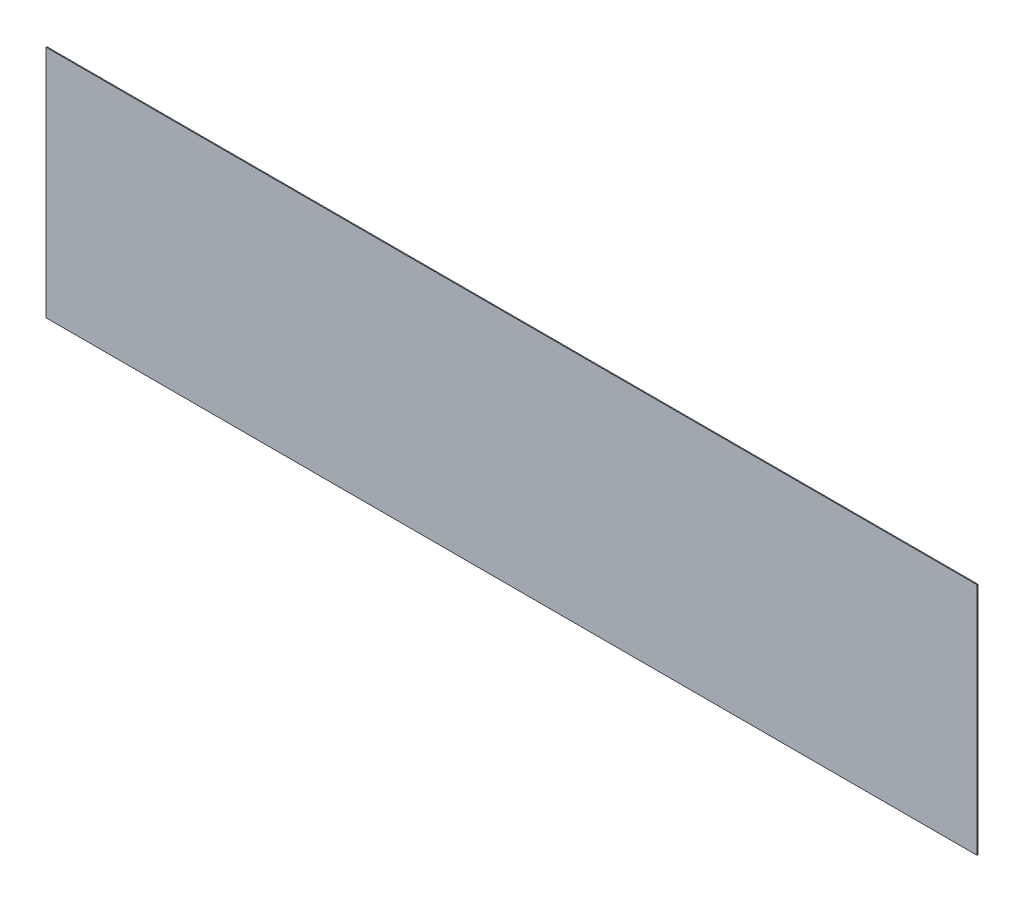
from build123d import *

# Parameters (mm, degrees)
SKETCH1_W           = 6000
SKETCH1_H           = 1510
BOSS_EXTRUDE1_DEPTH = 6


with BuildPart() as part:
    # Sketch1 → Boss-Extrude1 (new body)
    with BuildSketch(Plane.XY):
        with Locations((3000, 755)):
            Rectangle(SKETCH1_W, SKETCH1_H)
    extrude(amount=BOSS_EXTRUDE1_DEPTH)


solid = part.part
